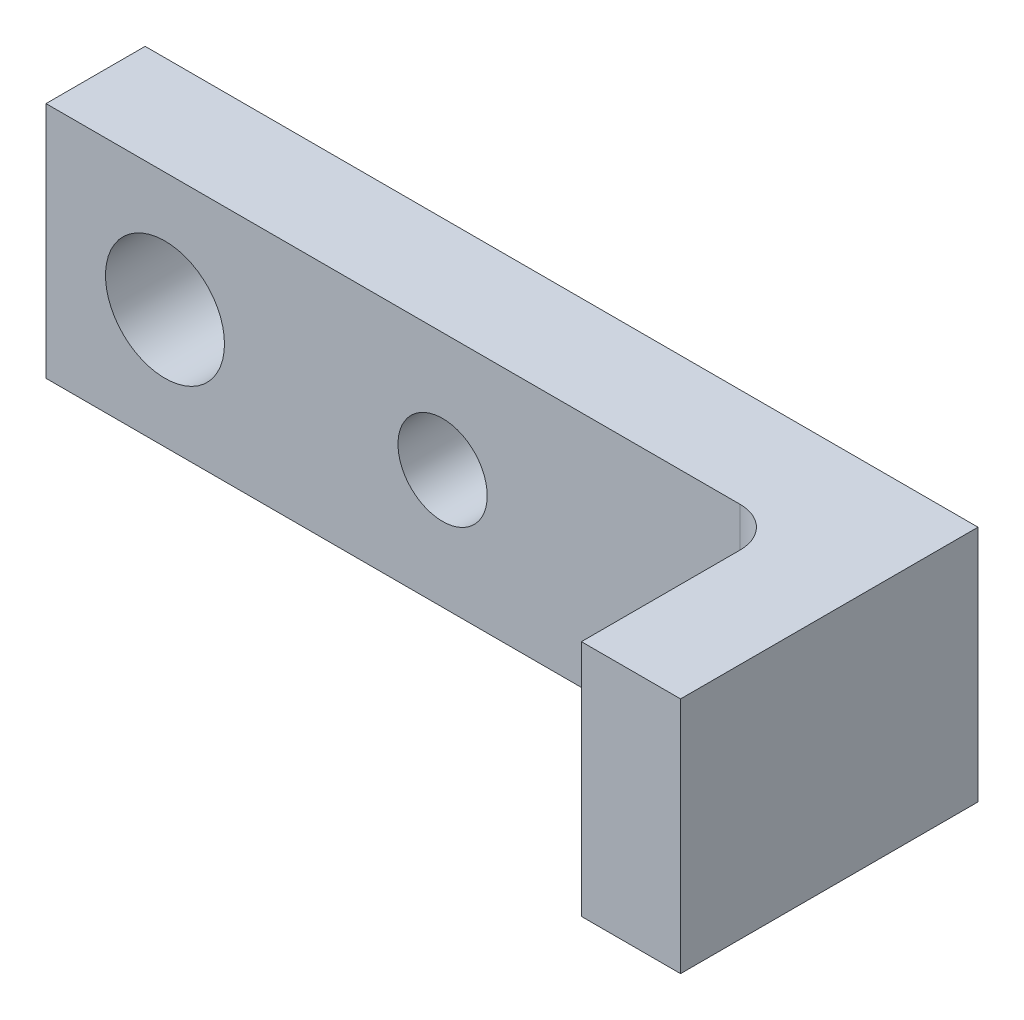
from build123d import *

# Parameters (mm, degrees)
SKETCH1_W           = 42
SKETCH1_H           = 12
SKETCH1_R           = 2.25
SKETCH1_R_2         = 3
BOSS_EXTRUDE1_DEPTH = 5
SKETCH2_W           = 5
SKETCH2_H           = 12
BOSS_EXTRUDE2_DEPTH = 10
FILLET1_R           = 2


with BuildPart() as part:
    # Sketch1 → Boss-Extrude1 (new body)
    with BuildSketch(Plane.XY):
        with Locations((21, 6)):
            Rectangle(SKETCH1_W, SKETCH1_H)
        with Locations((20, 6)):
            Circle(SKETCH1_R, mode=Mode.SUBTRACT)
        with Locations((6, 6)):
            Circle(SKETCH1_R_2, mode=Mode.SUBTRACT)
    extrude(amount=BOSS_EXTRUDE1_DEPTH)

    # Sketch2 → Boss-Extrude2 (add)
    with BuildSketch(Plane.XY.offset(5)):
        with Locations((39.5, 6)):
            Rectangle(SKETCH2_W, SKETCH2_H)
    extrude(amount=BOSS_EXTRUDE2_DEPTH)

    # Fillet1
    fillet1_edges = [part.edges().sort_by_distance(p)[0] for p in [
        (37, 6, 5),
    ]]
    fillet(fillet1_edges, radius=FILLET1_R)


solid = part.part
